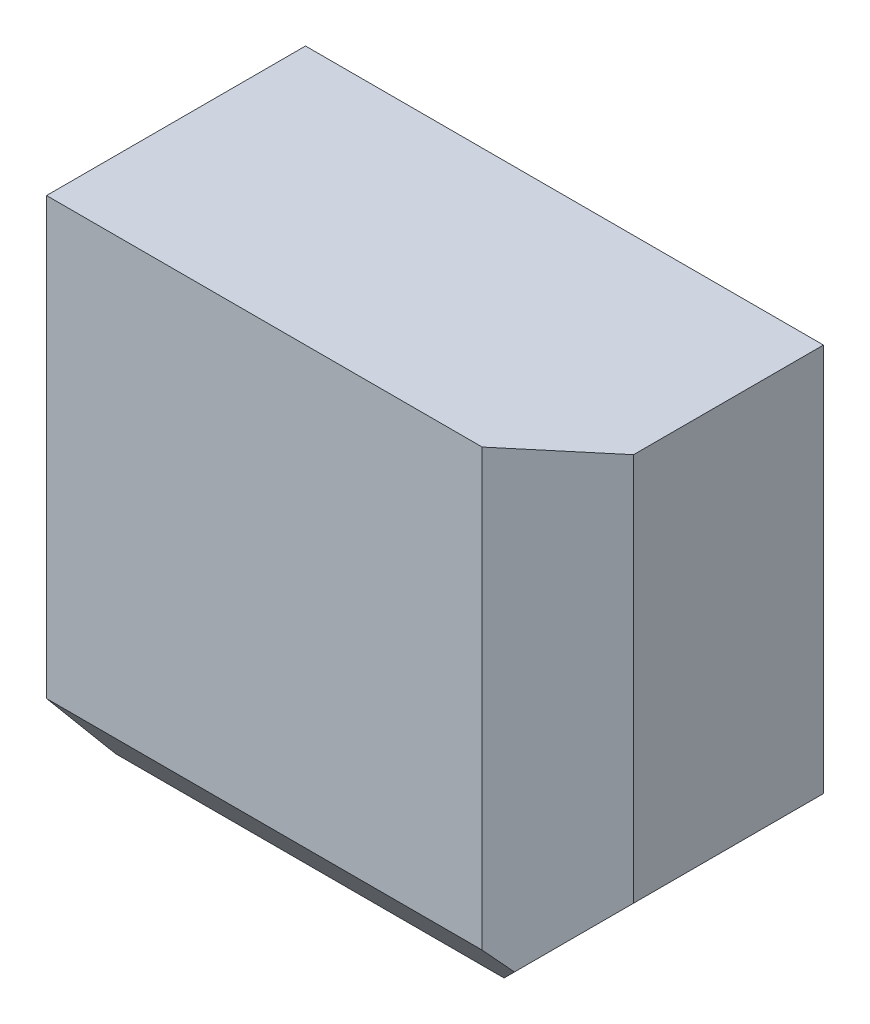
SolidWorks part; units mm, degrees
material "普通碳钢"
ref_plane "Front Plane" through (0, 0, 0) normal (0, 0, 1) x (1, 0, 0)
ref_plane "Top Plane" through (0, 0, 0) normal (0, 1, 0) x (1, 0, 0)
ref_plane "Right Plane" through (0, 0, 0) normal (1, 0, 0) x (0, 0, -1)
sketch "Sketch1" plane through (0, 0, 0) normal (0, 0, 1) x (1, 0, 0)
  line L1 (-30, 30) -> (30, 30)
  line L2 (-30, 30) -> (-30, -30)
  line L3 (-30, -30) -> (30, -30)
  line L4 (30, 30) -> (30, -30)
  dimension "D1" = 60
  dimension "D2" = 60
  dimension "D3" = 30
  dimension "D4" = 30
extrude "Boss-Extrude1" add sketch "Sketch1" along normal mid plane 30
chamfer "Chamfer1" distance 15 angle 45 1 edges at (30, -30, 0)
chamfer "Chamfer2" distance 8 angle 50 1 edges at (-7.5, -30, 15)
chamfer "Chamfer3" distance 8 angle 50 1 edges at (30, 7.5, 15)
